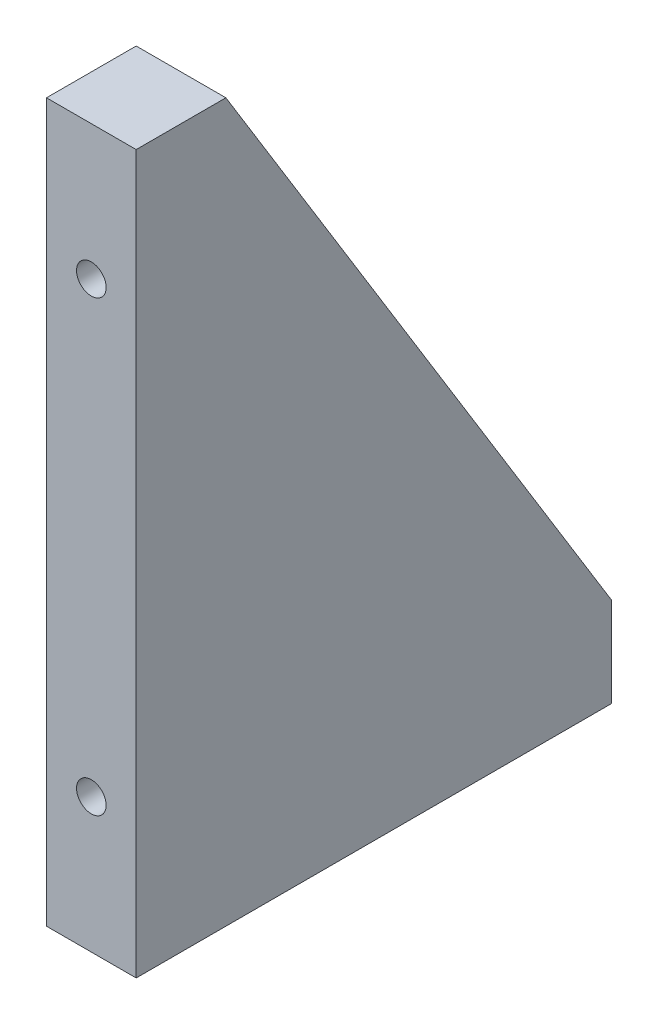
from build123d import *

# Parameters (mm, degrees)
BOSS_EXTRUDE1_DEPTH   = 10
M4_TAPPED_HOLE1_D     = 3.3
M4_TAPPED_HOLE1_DEPTH = 10.1
M4_TAPPED_HOLE1_TIP   = 0.991420021
M4_TAPPED_HOLE2_D     = 3.3
M4_TAPPED_HOLE2_DEPTH = 10.1
M4_TAPPED_HOLE2_TIP   = 0.991420021


with BuildPart() as part:
    # Sketch1 → Boss-Extrude1 (new body)
    with BuildSketch(Plane(origin=(0, 0, 0), x_dir=(0, 0, -1), z_dir=(1, 0, 0))):
        Polygon((0, 0), (0, 80), (10, 80), (53, 10), (53, 0), align=None)
    extrude(amount=BOSS_EXTRUDE1_DEPTH)

    # M4 Tapped Hole1
    with Locations(Plane.XY):
        with Locations((5, 65), (5, 15)):
            Hole(M4_TAPPED_HOLE1_D / 2, depth=M4_TAPPED_HOLE1_DEPTH)
            with Locations((0, 0, -(M4_TAPPED_HOLE1_DEPTH + M4_TAPPED_HOLE1_TIP / 2))):  # 118° drill point
                Cone(0, M4_TAPPED_HOLE1_D / 2, M4_TAPPED_HOLE1_TIP, mode=Mode.SUBTRACT)

    # M4 Tapped Hole2
    with Locations(Plane(origin=(0, 0, 0), x_dir=(-1, 0, 0), z_dir=(0, -1, 0))):
        with Locations((-5, 43), (-5, 8)):
            Hole(M4_TAPPED_HOLE2_D / 2, depth=M4_TAPPED_HOLE2_DEPTH)
            with Locations((0, 0, -(M4_TAPPED_HOLE2_DEPTH + M4_TAPPED_HOLE2_TIP / 2))):  # 118° drill point
                Cone(0, M4_TAPPED_HOLE2_D / 2, M4_TAPPED_HOLE2_TIP, mode=Mode.SUBTRACT)


solid = part.part
